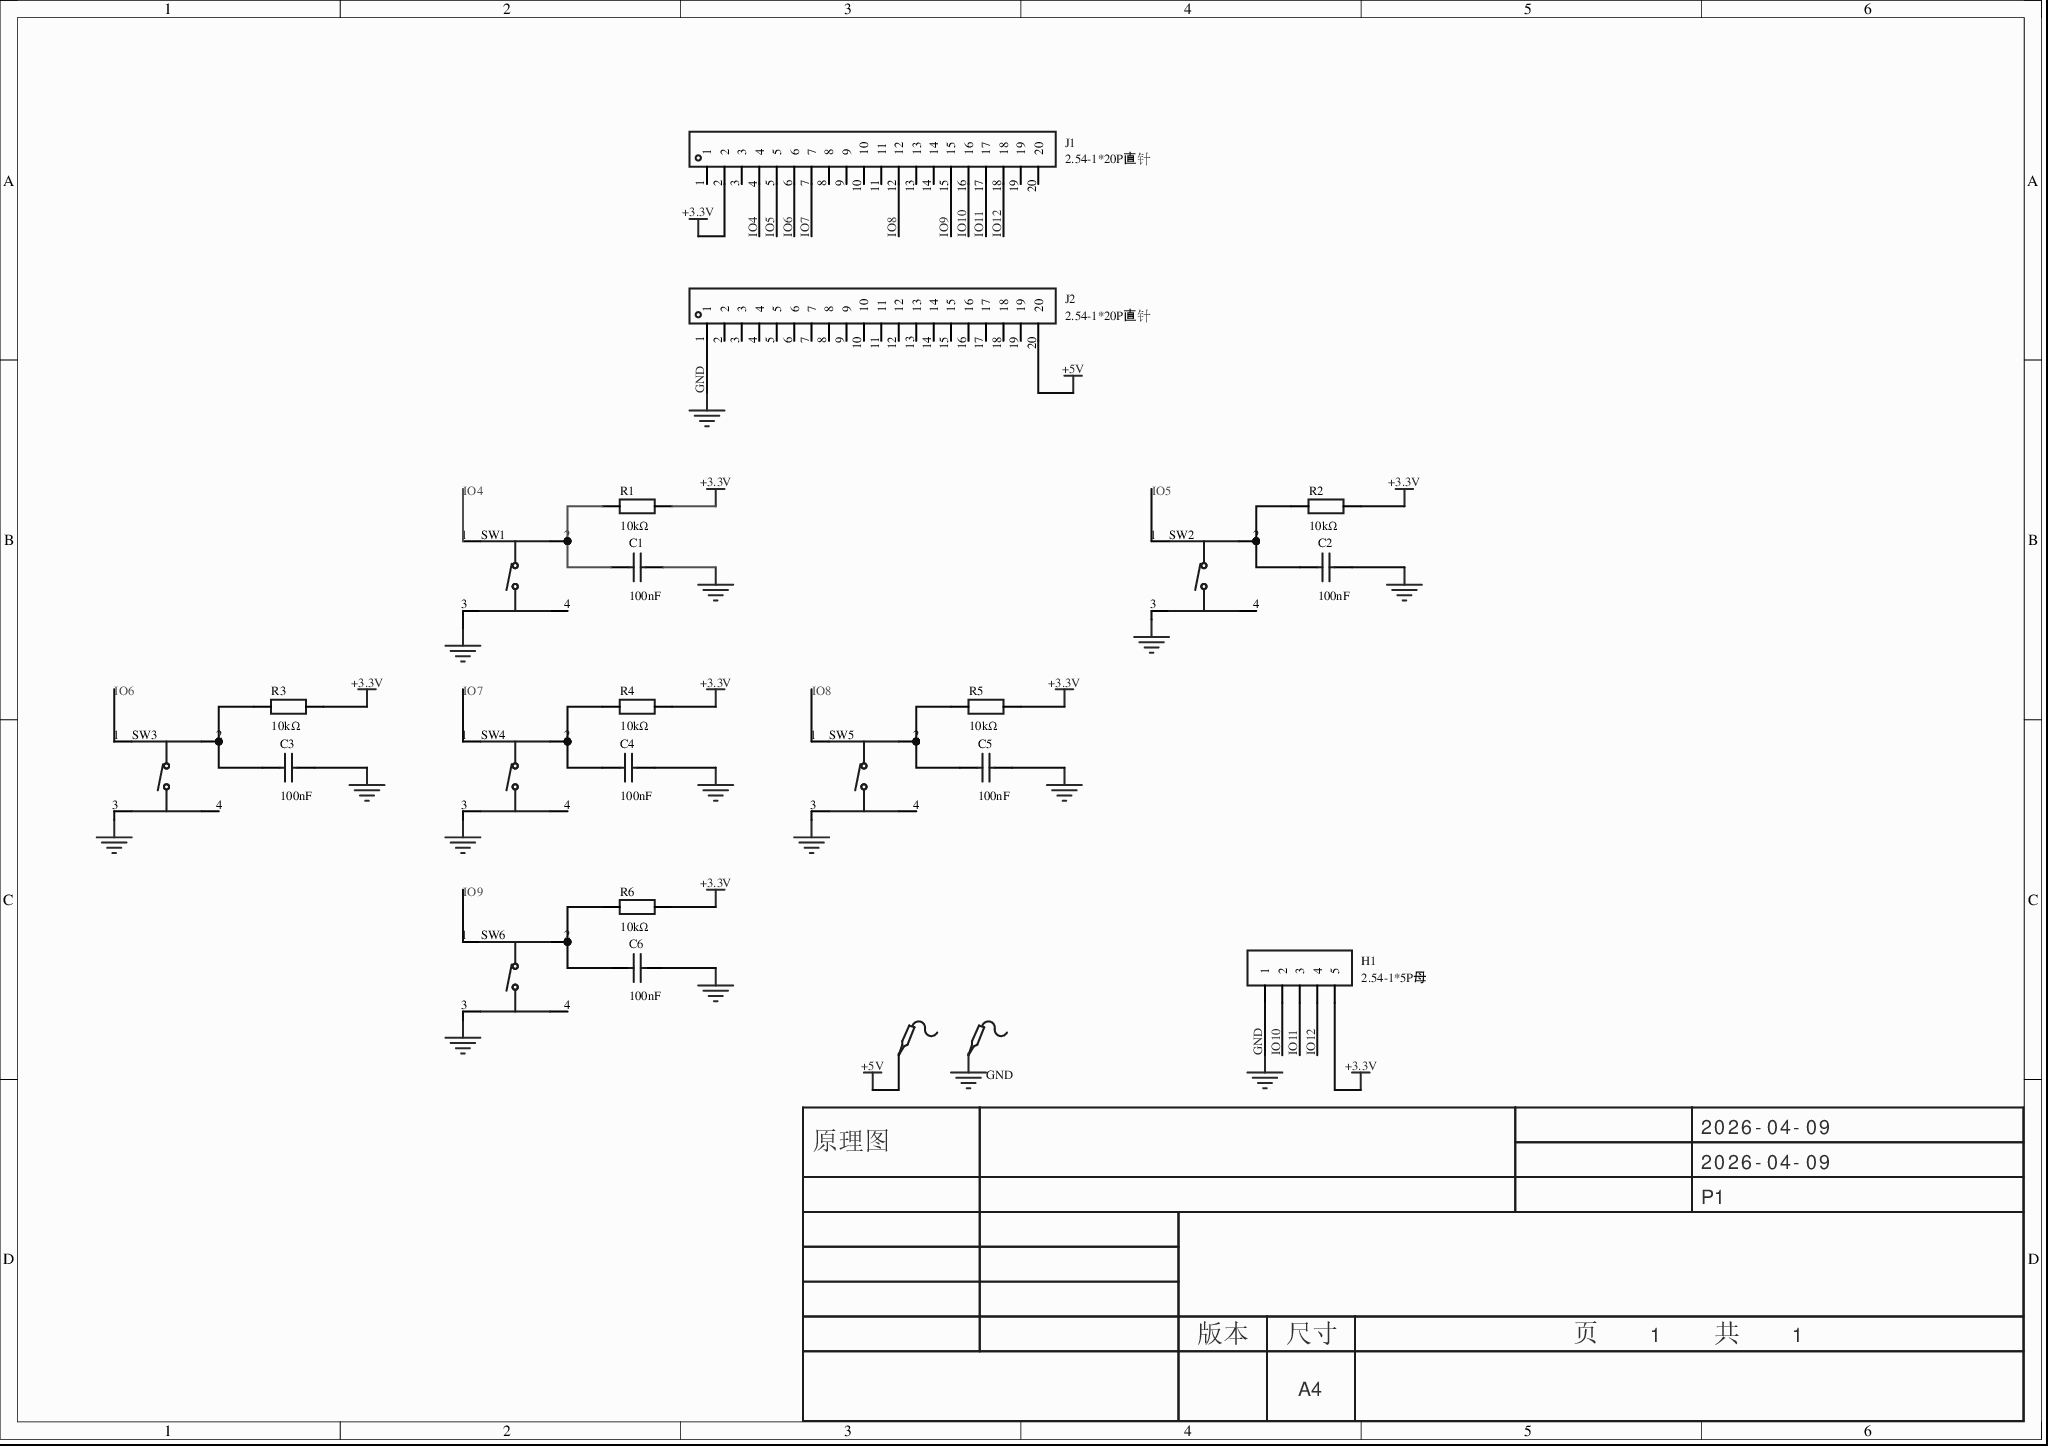
[diagram p0: MISC51976-3.schdoc]
# Altium project MISC51976-2.PrjPcb
1 sheet, 23 parts. Net scope: global (net labels, ports and power ports of the same name join across sheets).
Board file: MISC51976.pcbdoc

## Sheet MISC51976-3.schdoc
size 297 x 209 mm; Version: V1.0; @Project Name: MISC51976; @Update Date: 2026-04-09; @Create Date: 2026-04-09; @Board Name: MISC51976; @Create Time: 09:40:49; @Page Count: 1; @Page No: 1; @Schematic Name: MISC51976; @Update Time: 09:40:49; Size: A4

### Parts
5V  (no value)  [Test-Point-0.5mm]
C1  100nF  [C0805]
C2  100nF  [C0805]
C3  100nF  [C0805]
C4  100nF  [C0805]
C5  100nF  [C0805]
C6  100nF  [C0805]
GND  (no value)  [Test-Point-0.5mm]
H1  2.54-1*5P母  [HDR-TH_5P-P2.54-V-F]
J1  2.54-1*20P直针  [HDR-TH_20P-P2.54-V-M-1]
J2  2.54-1*20P直针  [HDR-TH_20P-P2.54-V-M-1]
R1  10kΩ  [R0805]
R2  10kΩ  [R0805]
R3  10kΩ  [R0805]
R4  10kΩ  [R0805]
R5  10kΩ  [R0805]
R6  10kΩ  [R0805]
SW1  TC-1103-C-K  [KEY-TH_4P-L12.0-W12.0-P5.00-LS12.5]  (value not drawn)
SW2  TC-1103-C-K  [KEY-TH_4P-L12.0-W12.0-P5.00-LS12.5]  (value not drawn)
SW3  TC-1103-C-K  [KEY-TH_4P-L12.0-W12.0-P5.00-LS12.5]  (value not drawn)
SW4  TC-1103-C-K  [KEY-TH_4P-L12.0-W12.0-P5.00-LS12.5]  (value not drawn)
SW5  TC-1103-C-K  [KEY-TH_4P-L12.0-W12.0-P5.00-LS12.5]  (value not drawn)
SW6  TC-1103-C-K  [KEY-TH_4P-L12.0-W12.0-P5.00-LS12.5]  (value not drawn)

### Nets
+3.3V: H1.5 J1.2 R1.2 R2.2 R3.2 R4.2 R5.2 R6.2
+5V: 5V.1 J2.20
GND: C1.2 C2.2 C3.2 C4.2 C5.2 C6.2 GND.1 H1.1 J2.1 SW1.3 SW2.3 SW3.3 SW4.3 SW5.3 SW6.3
IO4: J1.4 SW1.1
IO5: J1.5 SW2.1
IO6: J1.6 SW3.1
IO7: J1.7 SW4.1
IO8: J1.12 SW5.1
IO9: J1.15 SW6.1
IO10: H1.2 J1.16
IO11: H1.3 J1.17
IO12: H1.4 J1.18
NetC1_1: C1.1 R1.1 SW1.2
NetC2_1: C2.1 R2.1 SW2.2
NetC3_1: C3.1 R3.1 SW3.2
NetC4_1: C4.1 R4.1 SW4.2
NetC5_1: C5.1 R5.1 SW5.2
NetC6_1: C6.1 R6.1 SW6.2

Not connected (* = marked no-connect by the designer): J1 1 3 8 9 10 11 13 14 19 20; J2 2 3 4 5 6 7 8 9 10 11 12 13 14 15 16 17 18 19; SW1 4; SW2 4; SW3 4; SW4 4; SW5 4; SW6 4

### Notes on the sheet
- 2026-04-09
- 原理图
- P1
- 版本
- 尺寸
- A4
- 页    1    共    1

### Library data of the parts
5V GND = Test-Point: Check: false; AddInBom: yes; Symbol: Test-Point; Device: Test-Point; ConvertToPcb: yes; FootprintName: Test-Point-0.5mm; Description: Test-Point
C1-C6 = CC0805KKX7R0BB104: 容值:100nF;精度:±10%;额定电压:100V;材质(温度系数):X7R;; Manufacturer: YAGEO(国巨); Add into BOM: yes; 3D Model: 1ba041120af144c991958decab20d241; 3D Model Transform: 78.74,51.181,0,0,0,0,0,0.0005,0; Tolerance: ±10%; Temperature Coefficient: X7R; Voltage Rated: 100V; ModelName: C0805_L2.0-W1.3-H1.3; Symbol: CC0805KKX7R0BB104; Device: CC0805KKX7R0BB104; Convert to PCB: yes; LCSC Part Name: 100nF ±10% 100V; Supplier Part: C106243; Manufacturer Part: CC0805KKX7R0BB104; Supplier Footprint: 0805; JLCPCB Part Class: Extended Part; Datasheet: https://atta.szlcsc.com/upload/public/pdf/source/20170505/1493951378248.pdf; Supplier: LCSC; Value: 100nF; FootprintName: C0805
H1 = 2.54-1*5P母: 间距:2.54mm;总孔位数:5;排数:1;插孔结构:1x5P;行距:-;安装类型:直插;塑高:-;触头材质:-;触头镀层:-;; Manufacturer: BOOMELE(博穆精密); Symbol: Header-Female-2.54_1x5; AddInBom: yes; ModelId: fbeffe0d3b4a40f6888dab4bd9d4db880819f05c4eef4c71ace90d822a990e87; ModelName: HDR2.54-F-LI-1X5P; ModelTransform: 499.999,100,0,0,0,0,0,0,-118.11; Pitch: 2.54mm; Number of Holes: 5; Holes Structure: 1x5P; Device: 2.54-1*5P母; Supplier: LCSC; Manufacturer Part: 2.54-1*5P母; Supplier Part: C50950; JLCPCB Part Class: Extended Part; LCSC Part Name: 2.54mm 1x5P; Supplier Footprint: 直插,P=2.54mm; Datasheet: https://atta.szlcsc.com/upload/public/pdf/source/20151109/1457707571406.pdf; ConvertToPcb: yes; FootprintName: HDR-TH_5P-P2.54-V-F; Number of Rows: 1; Row Spacing: -; Mounting Type: 直插; Insulation Height: -; Contact Material: -; Contact Plating: -
J1 = 2.54-1*20P直针: 间距:2.54mm;总PIN位数:20;排数:1;插针结构:1x20P;行距:-;安装类型:直插;圆针/方针:方针;额定电流:3A;额定电压:-;配合针长度:-;塑高:-;端接针长度:-;触头材质:黄铜;触头镀层:-;工作温度范围:-40℃~+105℃;颜色:黑色;; Manufacturer: BOOMELE(博穆精密); Symbol: Header-Male-2.54_1x20; AddInBom: yes; ModelId: f68709be121d406db68b06f32a5953890819f05c4eef4c71ace90d822a990e87; ModelName: HDR-M-2.54_1x20; ModelTransform: 2000,100,0,0,0,0,0,2.5,-118.1; Pitch: 2.54mm; Pin Structure: 1x20P; Circluar Pins/Square Pins: 方针; Current Rating (Max): 3A; Device: 2.54-1*20P直针; LCSC Part Name: 2.54mm 1x20P 直插 方针; SupplierPart: C50981; ManufacturerPart: 2.54-1*20P直针; Supplier Footprint: 插件,P=2.54mm; JLCPCB Part Class: Extended Part; Datasheet: https://atta.szlcsc.com/upload/public/pdf/source/20151109/1457707571495.pdf; Supplier: LCSC; ConvertToPcb: yes; FootprintName: HDR-TH_20P-P2.54-V-M-1; Number of Pins: 20; Number of Rows: 1; Row Spacing: -; Mounting Type: 直插; Voltage Rating (Max): -; Length of Mating Pin: -; Insulation Height: -; Length of End Connection Pin: -; Contact Material: 黄铜; Contact Plating: -; Operating Temperature Range: -40℃~+105℃; Color: 黑色
J2 = 2.54-1*20P直针: 间距:2.54mm;总PIN位数:20;排数:1;插针结构:1x20P;行距:-;安装类型:直插;圆针/方针:方针;额定电流:3A;额定电压:-;配合针长度:-;塑高:-;端接针长度:-;触头材质:黄铜;触头镀层:-;工作温度范围:-40℃~+105℃;颜色:黑色;; Manufacturer: BOOMELE(博穆精密); Symbol: Header-Male-2.54_1x20; 3D Model: f68709be121d406db68b06f32a5953890819f05c4eef4c71ace90d822a990e87; 3D Model Transform: 2000,100,0,0,0,0,0,2.5,-118.1; Pitch: 2.54mm; Pin Structure: 1x20P; Circluar Pins/Square Pins: 方针; Current Rating (Max): 3A; AddInBom: yes; ModelName: HDR-M-2.54_1x20; Device: 2.54-1*20P直针; LCSC Part Name: 2.54mm 1x20P 直插 方针; Supplier Part: C50981; Manufacturer Part: 2.54-1*20P直针; Supplier Footprint: 插件,P=2.54mm; JLCPCB Part Class: Extended Part; Datasheet: https://atta.szlcsc.com/upload/public/pdf/source/20151109/1457707571495.pdf; Supplier: LCSC; Number of Pins: 20; Number of Rows: 1; Row Spacing: -; Mounting Type: 直插; Voltage Rating (Max): -; Length of Mating Pin: -; Insulation Height: -; Length of End Connection Pin: -; Contact Material: 黄铜; Contact Plating: -; Operating Temperature Range: -40℃~+105℃; Color: 黑色; ConvertToPcb: yes; FootprintName: HDR-TH_20P-P2.54-V-M-1
R1-R6 = CR0805J80103G: 电阻类型:厚膜电阻;阻值:10kΩ;精度:±5%;功率:125mW;温度系数:±200ppm/℃;最大工作电压:150V;工作温度范围:-55℃~+125℃;; Manufacturer: LIZ(丽智电子); Add into BOM: yes; 3D Model: 37a81e68749a4138bd2dfa6897b24b85; 3D Model Transform: 78.74,51.181,0,0,0,0,0,-0.0005,0; Tolerance: ±5%; Power(Watts): 125mW; Overload Voltage (Max): 150V; ModelName: R0805_L2.0-W1.3-H0.6; Symbol: CR0805J80103G; Device: CR0805J80103G; Convert to PCB: yes; LCSC Part Name: 10kΩ ±5% 125mW; Supplier Part: C101926; Manufacturer Part: CR0805J80103G; Supplier Footprint: 0805; JLCPCB Part Class: Extended Part; Datasheet: https://atta.szlcsc.com/upload/public/pdf/source/20170408/1491635765379.pdf; Supplier: LCSC; Type: 厚膜电阻; Value: 10kΩ; Temperature Coefficient: ±200ppm/℃; Operating Temperature Range: -55℃~+125℃; FootprintName: R0805
SW1-SW6 = TC-1103-C-K: 触点电流:50mA;额定电压(DC):12V;绝缘电阻:100mΩ;电路结构:单刀单掷;安装方式:直插;按钮形状:圆形按钮;按钮/盖帽颜色:黑色;带灯:无;作用力:260gf;机械寿命:100000;工作温度:-30℃~+85℃;引脚样式:PC引脚;开关长度:12mm;开关宽度:12mm;开关高度:9mm;带支架:否;; Manufacturer: XKB Connectivity(中国星坤); Add into BOM: yes; 3D Model: 58bd23e2e6df4c6ea4917606aab27058; 3D Model Transform: 543,472.4,0,0,0,0,0,0,-137.8; Contact Current: 50mA; Voltage Rating (DC): 12V; Insulation Resistance: 100mΩ; Circuit: 单刀单掷; Actuator Style: 圆形按钮; Actuator/Cap Color: 黑色; With Lamp: 无; Operating Force: 260gf; Mechanical Life: 100000; Pin Style: PC引脚; Switch Length: 12mm; Switch Height: 9mm; Strike Gundam: 否; Symbol: TC-1103-C-K; Device: TC-1103-C-K; Convert to PCB: yes; Supplier Part: C318972; Supplier Footprint: 插件; LCSC Part Name: 12*12*9.0 圆柱 250gf; Manufacturer Part: TC-1103-C-K; JLCPCB Part Class: Extended Part; Datasheet: https://atta.szlcsc.com/upload/public/pdf/source/20211011/68D1180622A7471600864EE2962EC968.pdf; Supplier: LCSC; Mounting Style: 直插; Operating Temperature: -30℃~+85℃; Switch Width: 12mm; FootprintName: KEY-TH_4P-L12.0-W12.0-P5.00-LS12.5; ModelName: KEY-TH_4P-L12.0-W12.0-P5.00-LS12.5